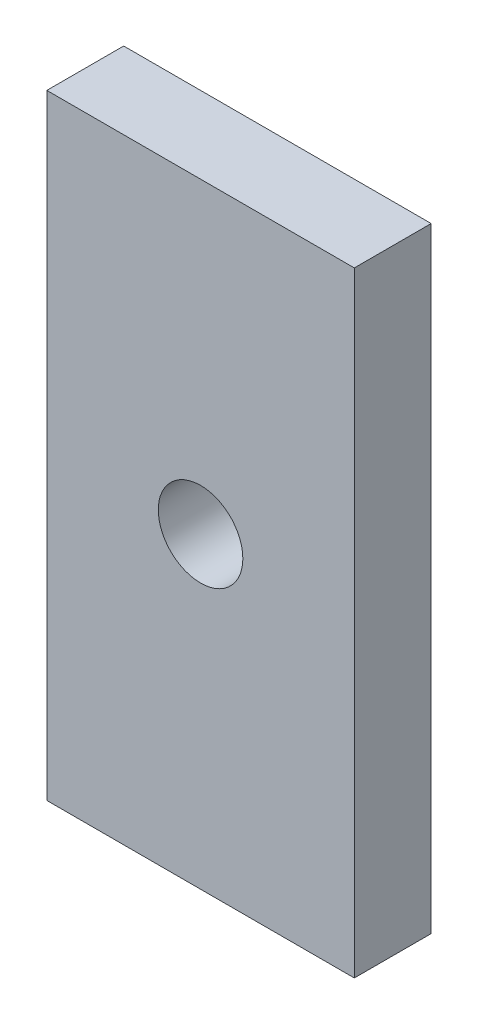
from build123d import *

# Parameters (mm, degrees)
SKETCH1_W                  = 40
SKETCH1_H                  = 80
BOSS_EXTRUDE1_DEPTH        = 10
F_11_0_11_DIAMETER_HOLE1_D = 11


with BuildPart() as part:
    # Sketch1 → Boss-Extrude1 (new body)
    with BuildSketch(Plane.XY):
        with Locations((20, 40)):
            Rectangle(SKETCH1_W, SKETCH1_H)
    extrude(amount=BOSS_EXTRUDE1_DEPTH)

    # Ø11.0 (11) Diameter Hole1 (through all)
    with Locations(Plane.XY.offset(10)):
        with Locations((20, 40)):
            Hole(F_11_0_11_DIAMETER_HOLE1_D / 2)


solid = part.part
